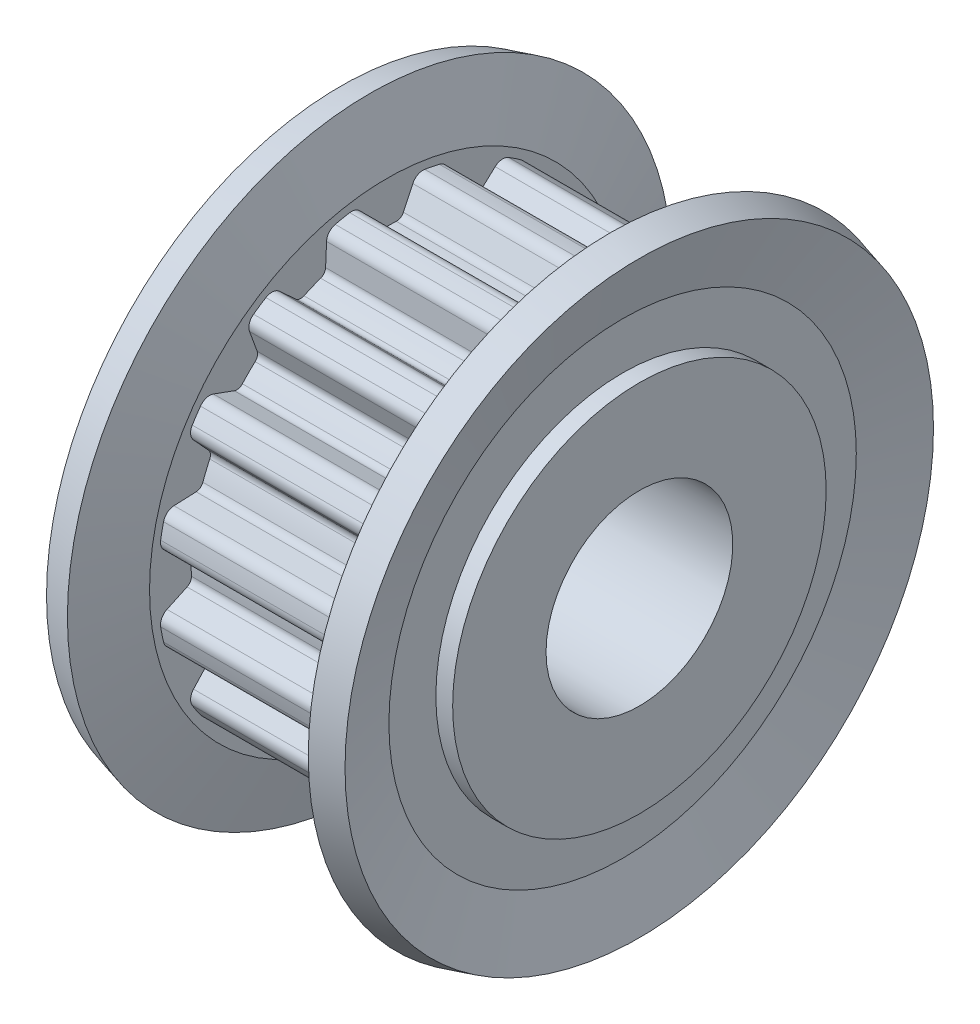
SolidWorks part; units mm, degrees
ref_plane "前视" through (0, 0, 0) normal (0, 0, 1) x (1, 0, 0)
ref_plane "上视" through (0, 0, 0) normal (0, 1, 0) x (1, 0, 0)
ref_plane "右视" through (0, 0, 0) normal (1, 0, 0) x (0, 0, -1)
sketch "草图1" plane through (0, 0, 0) normal (0, 0, 1) x (1, 0, 0)
  line L0 (0, 9.8) -> (0, 5.2)
  line L1 (0, 5.2) -> (0.2, 5)
  line L2 (0.2, 5) -> (16, 5)
  line L3 (16, 5) -> (16, 10)
  line L4 (16, 10) -> (15.1, 10)
  line L5 (15.1, 10) -> (15.1, 12.5138)
  line L6 (15.1, 12.5138) -> (15.9919, 15.7545)
  line L7 (15.9919, 15.7545) -> (14.4493, 16.1791)
  line L8 (14.4493, 16.1791) -> (13.5, 12.73)
  line L9 (13.5, 12.73) -> (2.5, 12.73)
  line L10 (2.5, 12.73) -> (1.5507, 16.1791)
  line L11 (1.5507, 16.1791) -> (0.0081, 15.7545)
  line L12 (0.0081, 15.7545) -> (0.9, 12.5138)
  line L13 (0.9, 12.5138) -> (0.9, 10)
  line L14 (0.9, 10) -> (0.2, 10)
  line L15 (0.2, 10) -> (0, 9.8)
  line L16 (28, 0) -> (0, 0) construction
revolve "旋转1" add sketch "草图1" angle 360 about L16
ref_plane "基准面1" through (2.5, 0, 0) normal (1, 0, 0) x (0, 0, -1)
sketch "草图2" plane through (2.5, 0, 0) normal (1, 0, 0) x (0, 0, -1)
  line L0 (-32, -32) -> (32, -32)
  line L1 (32, -32) -> (32, 32)
  line L2 (32, 32) -> (-32, 32)
  line L3 (-32, 32) -> (-32, -32)
  line L4 (-11.4217, -3.2513) -> (-10.2344, -3.3032)
  line L5 (-9.5725, -4.9011) -> (-10.3754, -5.7773)
  line L6 (-9.308, -7.3747) -> (-8.1912, -6.9682)
  line L7 (-6.9682, -8.1912) -> (-7.3747, -9.308)
  line L8 (-5.7773, -10.3754) -> (-4.9011, -9.5725)
  line L9 (-3.3032, -10.2344) -> (-3.2513, -11.4217)
  line L10 (-1.3671, -11.7965) -> (-0.8648, -10.7194)
  line L11 (0.8648, -10.7194) -> (1.3671, -11.7965)
  line L12 (3.2513, -11.4217) -> (3.3032, -10.2344)
  line L13 (4.9011, -9.5725) -> (5.7773, -10.3754)
  line L14 (7.3747, -9.308) -> (6.9682, -8.1912)
  line L15 (8.1912, -6.9682) -> (9.308, -7.3747)
  line L16 (10.3754, -5.7773) -> (9.5725, -4.9011)
  line L17 (10.2344, -3.3032) -> (11.4217, -3.2513)
  line L18 (11.7965, -1.3671) -> (10.7194, -0.8648)
  line L19 (10.7194, 0.8648) -> (11.7965, 1.3671)
  line L20 (11.4217, 3.2513) -> (10.2344, 3.3032)
  line L21 (9.5725, 4.9011) -> (10.3754, 5.7773)
  line L22 (9.308, 7.3747) -> (8.1912, 6.9682)
  line L23 (6.9682, 8.1912) -> (7.3747, 9.308)
  line L24 (5.7773, 10.3754) -> (4.9011, 9.5725)
  line L25 (3.3032, 10.2344) -> (3.2513, 11.4217)
  line L26 (1.3671, 11.7965) -> (0.8648, 10.7194)
  line L27 (-0.8648, 10.7194) -> (-1.3671, 11.7965)
  line L28 (-3.2513, 11.4217) -> (-3.3032, 10.2344)
  line L29 (-4.9011, 9.5725) -> (-5.7773, 10.3754)
  line L30 (-7.3747, 9.308) -> (-6.9682, 8.1912)
  line L31 (-8.1912, 6.9682) -> (-9.308, 7.3747)
  line L32 (-10.3754, 5.7773) -> (-9.5725, 4.9011)
  line L33 (-10.2344, 3.3032) -> (-11.4217, 3.2513)
  line L34 (-11.7965, 1.3671) -> (-10.7194, 0.8648)
  line L35 (-10.7194, -0.8648) -> (-11.7965, -1.3671)
  arc A0 (-11.7965, -1.3671) -> (-12.1348, -2.0088) centre (-11.5429, -1.9108) ccw
  arc A1 (-12.1348, -2.0088) -> (-12.0637, -2.3996) centre (0, 0) ccw
  arc A2 (-12.0637, -2.3996) -> (-11.9799, -2.7879) centre (0, 0) ccw
  arc A3 (-11.9799, -2.7879) -> (-11.4217, -3.2513) centre (-11.3955, -2.6519) ccw
  arc A4 (-10.2344, -3.3032) -> (-9.8756, -3.5669) centre (-10.2518, -3.7028) cw
  arc A5 (-9.8756, -3.5669) -> (-9.5053, -4.4609) centre (0, 0) ccw
  arc A6 (-9.5053, -4.4609) -> (-9.5725, -4.9011) centre (-9.8674, -4.6309) cw
  arc A7 (-10.3754, -5.7773) -> (-10.4424, -6.4997) centre (-9.933, -6.1827) ccw
  arc A8 (-10.4424, -6.4997) -> (-10.2271, -6.8335) centre (0, 0) ccw
  arc A9 (-10.2271, -6.8335) -> (-10.0011, -7.1602) centre (0, 0) ccw
  arc A10 (-10.0011, -7.1602) -> (-9.308, -7.3747) centre (-9.5132, -6.8109) ccw
  arc A11 (-8.1912, -6.9682) -> (-7.7589, -7.0746) centre (-8.0544, -7.3441) cw
  arc A12 (-7.7589, -7.0746) -> (-7.0746, -7.7589) centre (0, 0) ccw
  arc A13 (-7.0746, -7.7589) -> (-6.9682, -8.1912) centre (-7.3441, -8.0544) cw
  arc A14 (-7.3747, -9.308) -> (-7.1602, -10.0011) centre (-6.8109, -9.5132) ccw
  arc A15 (-7.1602, -10.0011) -> (-6.8335, -10.2271) centre (0, 0) ccw
  arc A16 (-6.8335, -10.2271) -> (-6.4997, -10.4424) centre (0, 0) ccw
  arc A17 (-6.4997, -10.4424) -> (-5.7773, -10.3754) centre (-6.1827, -9.933) ccw
  arc A18 (-4.9011, -9.5725) -> (-4.4609, -9.5053) centre (-4.6309, -9.8674) cw
  arc A19 (-4.4609, -9.5053) -> (-3.5669, -9.8756) centre (0, 0) ccw
  arc A20 (-3.5669, -9.8756) -> (-3.3032, -10.2344) centre (-3.7028, -10.2518) cw
  arc A21 (-3.2513, -11.4217) -> (-2.7879, -11.9799) centre (-2.6519, -11.3955) ccw
  arc A22 (-2.7879, -11.9799) -> (-2.3996, -12.0637) centre (0, 0) ccw
  arc A23 (-2.3996, -12.0637) -> (-2.0088, -12.1348) centre (0, 0) ccw
  arc A24 (-2.0088, -12.1348) -> (-1.3671, -11.7965) centre (-1.9108, -11.5429) ccw
  arc A25 (-0.8648, -10.7194) -> (-0.4838, -10.4888) centre (-0.5023, -10.8884) cw
  arc A26 (-0.4838, -10.4888) -> (0.4838, -10.4888) centre (0, 0) ccw
  arc A27 (0.4838, -10.4888) -> (0.8648, -10.7194) centre (0.5023, -10.8884) cw
  arc A28 (1.3671, -11.7965) -> (2.0088, -12.1348) centre (1.9108, -11.5429) ccw
  arc A29 (2.0088, -12.1348) -> (2.3996, -12.0637) centre (0, 0) ccw
  arc A30 (2.3996, -12.0637) -> (2.7879, -11.9799) centre (0, 0) ccw
  arc A31 (2.7879, -11.9799) -> (3.2513, -11.4217) centre (2.6519, -11.3955) ccw
  arc A32 (3.3032, -10.2344) -> (3.5669, -9.8756) centre (3.7028, -10.2518) cw
  arc A33 (3.5669, -9.8756) -> (4.4609, -9.5053) centre (0, 0) ccw
  arc A34 (4.4609, -9.5053) -> (4.9011, -9.5725) centre (4.6309, -9.8674) cw
  arc A35 (5.7773, -10.3754) -> (6.4997, -10.4424) centre (6.1827, -9.933) ccw
  arc A36 (6.4997, -10.4424) -> (6.8335, -10.2271) centre (0, 0) ccw
  arc A37 (6.8335, -10.2271) -> (7.1602, -10.0011) centre (0, 0) ccw
  arc A38 (7.1602, -10.0011) -> (7.3747, -9.308) centre (6.8109, -9.5132) ccw
  arc A39 (6.9682, -8.1912) -> (7.0746, -7.7589) centre (7.3441, -8.0544) cw
  arc A40 (7.0746, -7.7589) -> (7.7589, -7.0746) centre (0, 0) ccw
  arc A41 (7.7589, -7.0746) -> (8.1912, -6.9682) centre (8.0544, -7.3441) cw
  arc A42 (9.308, -7.3747) -> (10.0011, -7.1602) centre (9.5132, -6.8109) ccw
  arc A43 (10.0011, -7.1602) -> (10.2271, -6.8335) centre (0, 0) ccw
  arc A44 (10.2271, -6.8335) -> (10.4424, -6.4997) centre (0, 0) ccw
  arc A45 (10.4424, -6.4997) -> (10.3754, -5.7773) centre (9.933, -6.1827) ccw
  arc A46 (9.5725, -4.9011) -> (9.5053, -4.4609) centre (9.8674, -4.6309) cw
  arc A47 (9.5053, -4.4609) -> (9.8756, -3.5669) centre (0, 0) ccw
  arc A48 (9.8756, -3.5669) -> (10.2344, -3.3032) centre (10.2518, -3.7028) cw
  arc A49 (11.4217, -3.2513) -> (11.9799, -2.7879) centre (11.3955, -2.6519) ccw
  arc A50 (11.9799, -2.7879) -> (12.0637, -2.3996) centre (0, 0) ccw
  arc A51 (12.0637, -2.3996) -> (12.1348, -2.0088) centre (0, 0) ccw
  arc A52 (12.1348, -2.0088) -> (11.7965, -1.3671) centre (11.5429, -1.9108) ccw
  arc A53 (10.7194, -0.8648) -> (10.4888, -0.4838) centre (10.8884, -0.5023) cw
  arc A54 (10.4888, -0.4838) -> (10.4888, 0.4838) centre (0, 0) ccw
  arc A55 (10.4888, 0.4838) -> (10.7194, 0.8648) centre (10.8884, 0.5023) cw
  arc A56 (11.7965, 1.3671) -> (12.1348, 2.0088) centre (11.5429, 1.9108) ccw
  arc A57 (12.1348, 2.0088) -> (12.0637, 2.3996) centre (0, 0) ccw
  arc A58 (12.0637, 2.3996) -> (11.9799, 2.7879) centre (0, 0) ccw
  arc A59 (11.9799, 2.7879) -> (11.4217, 3.2513) centre (11.3955, 2.6519) ccw
  arc A60 (10.2344, 3.3032) -> (9.8756, 3.5669) centre (10.2518, 3.7028) cw
  arc A61 (9.8756, 3.5669) -> (9.5053, 4.4609) centre (0, 0) ccw
  arc A62 (9.5053, 4.4609) -> (9.5725, 4.9011) centre (9.8674, 4.6309) cw
  arc A63 (10.3754, 5.7773) -> (10.4424, 6.4997) centre (9.933, 6.1827) ccw
  arc A64 (10.4424, 6.4997) -> (10.2271, 6.8335) centre (0, 0) ccw
  arc A65 (10.2271, 6.8335) -> (10.0011, 7.1602) centre (0, 0) ccw
  arc A66 (10.0011, 7.1602) -> (9.308, 7.3747) centre (9.5132, 6.8109) ccw
  arc A67 (8.1912, 6.9682) -> (7.7589, 7.0746) centre (8.0544, 7.3441) cw
  arc A68 (7.7589, 7.0746) -> (7.0746, 7.7589) centre (0, 0) ccw
  arc A69 (7.0746, 7.7589) -> (6.9682, 8.1912) centre (7.3441, 8.0544) cw
  arc A70 (7.3747, 9.308) -> (7.1602, 10.0011) centre (6.8109, 9.5132) ccw
  arc A71 (7.1602, 10.0011) -> (6.8335, 10.2271) centre (0, 0) ccw
  arc A72 (6.8335, 10.2271) -> (6.4997, 10.4424) centre (0, 0) ccw
  arc A73 (6.4997, 10.4424) -> (5.7773, 10.3754) centre (6.1827, 9.933) ccw
  arc A74 (4.9011, 9.5725) -> (4.4609, 9.5053) centre (4.6309, 9.8674) cw
  arc A75 (4.4609, 9.5053) -> (3.5669, 9.8756) centre (0, 0) ccw
  arc A76 (3.5669, 9.8756) -> (3.3032, 10.2344) centre (3.7028, 10.2518) cw
  arc A77 (3.2513, 11.4217) -> (2.7879, 11.9799) centre (2.6519, 11.3955) ccw
  arc A78 (2.7879, 11.9799) -> (2.3996, 12.0637) centre (0, 0) ccw
  arc A79 (2.3996, 12.0637) -> (2.0088, 12.1348) centre (0, 0) ccw
  arc A80 (2.0088, 12.1348) -> (1.3671, 11.7965) centre (1.9108, 11.5429) ccw
  arc A81 (0.8648, 10.7194) -> (0.4838, 10.4888) centre (0.5023, 10.8884) cw
  arc A82 (0.4838, 10.4888) -> (-0.4838, 10.4888) centre (0, 0) ccw
  arc A83 (-0.4838, 10.4888) -> (-0.8648, 10.7194) centre (-0.5023, 10.8884) cw
  arc A84 (-1.3671, 11.7965) -> (-2.0088, 12.1348) centre (-1.9108, 11.5429) ccw
  arc A85 (-2.0088, 12.1348) -> (-2.3996, 12.0637) centre (0, 0) ccw
  arc A86 (-2.3996, 12.0637) -> (-2.7879, 11.9799) centre (0, 0) ccw
  arc A87 (-2.7879, 11.9799) -> (-3.2513, 11.4217) centre (-2.6519, 11.3955) ccw
  arc A88 (-3.3032, 10.2344) -> (-3.5669, 9.8756) centre (-3.7028, 10.2518) cw
  arc A89 (-3.5669, 9.8756) -> (-4.4609, 9.5053) centre (0, 0) ccw
  arc A90 (-4.4609, 9.5053) -> (-4.9011, 9.5725) centre (-4.6309, 9.8674) cw
  arc A91 (-5.7773, 10.3754) -> (-6.4997, 10.4424) centre (-6.1827, 9.933) ccw
  arc A92 (-6.4997, 10.4424) -> (-6.8335, 10.2271) centre (0, 0) ccw
  arc A93 (-6.8335, 10.2271) -> (-7.1602, 10.0011) centre (0, 0) ccw
  arc A94 (-7.1602, 10.0011) -> (-7.3747, 9.308) centre (-6.8109, 9.5132) ccw
  arc A95 (-6.9682, 8.1912) -> (-7.0746, 7.7589) centre (-7.3441, 8.0544) cw
  arc A96 (-7.0746, 7.7589) -> (-7.7589, 7.0746) centre (0, 0) ccw
  arc A97 (-7.7589, 7.0746) -> (-8.1912, 6.9682) centre (-8.0544, 7.3441) cw
  arc A98 (-9.308, 7.3747) -> (-10.0011, 7.1602) centre (-9.5132, 6.8109) ccw
  arc A99 (-10.0011, 7.1602) -> (-10.2271, 6.8335) centre (0, 0) ccw
  arc A100 (-10.2271, 6.8335) -> (-10.4424, 6.4997) centre (0, 0) ccw
  arc A101 (-10.4424, 6.4997) -> (-10.3754, 5.7773) centre (-9.933, 6.1827) ccw
  arc A102 (-9.5725, 4.9011) -> (-9.5053, 4.4609) centre (-9.8674, 4.6309) cw
  arc A103 (-9.5053, 4.4609) -> (-9.8756, 3.5669) centre (0, 0) ccw
  arc A104 (-9.8756, 3.5669) -> (-10.2344, 3.3032) centre (-10.2518, 3.7028) cw
  arc A105 (-11.4217, 3.2513) -> (-11.9799, 2.7879) centre (-11.3955, 2.6519) ccw
  arc A106 (-11.9799, 2.7879) -> (-12.0637, 2.3996) centre (0, 0) ccw
  arc A107 (-12.0637, 2.3996) -> (-12.1348, 2.0088) centre (0, 0) ccw
  arc A108 (-12.1348, 2.0088) -> (-11.7965, 1.3671) centre (-11.5429, 1.9108) ccw
  arc A109 (-10.7194, 0.8648) -> (-10.4888, 0.4838) centre (-10.8884, 0.5023) cw
  arc A110 (-10.4888, 0.4838) -> (-10.4888, -0.4838) centre (0, 0) ccw
  arc A111 (-10.4888, -0.4838) -> (-10.7194, -0.8648) centre (-10.8884, -0.5023) cw
extrude "切除-拉伸1" cut sketch "草图2" along normal blind 11
ref_plane "基准面2" through (8, 0, 0) normal (1, 0, 0) x (0, 0, -1)
